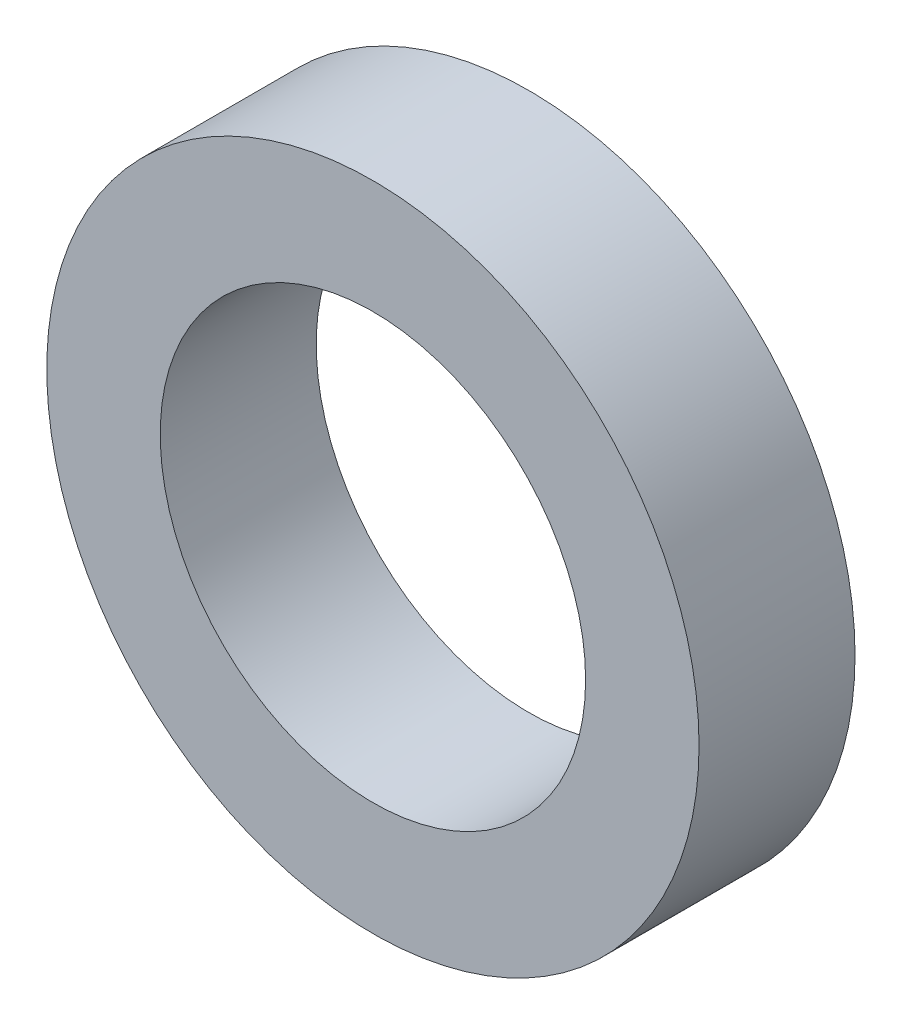
from build123d import *

# Parameters (mm, degrees)
SKETCH1_R           = 46
SKETCH1_R_2         = 30
BOSS_EXTRUDE1_DEPTH = 22


with BuildPart() as part:
    # Sketch1 → Boss-Extrude1 (new body)
    with BuildSketch(Plane.XY):
        Circle(SKETCH1_R)
        Circle(SKETCH1_R_2, mode=Mode.SUBTRACT)
    extrude(amount=BOSS_EXTRUDE1_DEPTH)


solid = part.part
